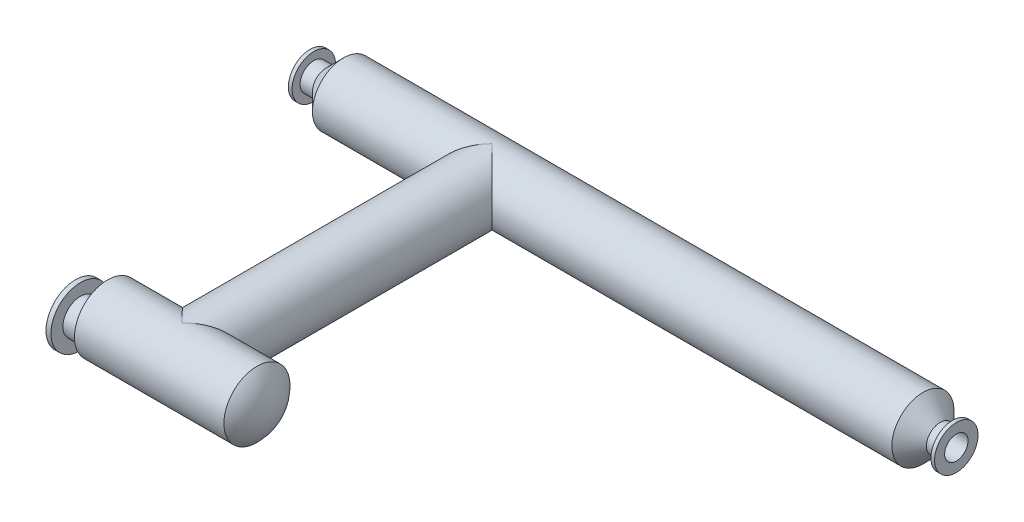
SolidWorks part; units mm, degrees
material "普通碳钢"
ref_plane "Front Plane" through (0, 0, 0) normal (0, 0, 1) x (1, 0, 0)
ref_plane "Top Plane" through (0, 0, 0) normal (0, 1, 0) x (1, 0, 0)
ref_plane "Right Plane" through (0, 0, 0) normal (1, 0, 0) x (0, 0, -1)
sketch "Sketch1" plane through (0, 0, 0) normal (0, 0, 1) x (1, 0, 0)
  line L0 (0, 56.5) -> (0, 105)
  line L1 (0, 105) -> (18, 105)
  line L2 (18, 105) -> (18, 66.5)
  line L3 (18, 66.5) -> (78, 66.5)
  line L4 (78, 66.5) -> (161.5, 150)
  line L5 (161.5, 150) -> (2962.5, 150)
  line L6 (2962.5, 150) -> (3046, 66.5)
  line L7 (3046, 66.5) -> (3106, 66.5)
  line L8 (3106, 66.5) -> (3106, 105)
  line L9 (3106, 105) -> (3124, 105)
  line L10 (3124, 105) -> (3124, 56.5)
  line L11 (3124, 56.5) -> (3041.8579, 56.5)
  line L12 (3041.8579, 56.5) -> (2958.3579, 140)
  line L13 (2958.3579, 140) -> (165.6421, 140)
  line L14 (165.6421, 140) -> (82.1421, 56.5)
  line L15 (82.1421, 56.5) -> (0, 56.5)
  line L16 (0, 0) -> (508.1939, 0) construction
  dimension "D1" = 3124
  dimension "D2" = 105
  dimension "D3" = 150
  dimension "D4" = 66.5
  dimension "D5" = 10
  dimension "D6" = 45
  dimension "D7" = 18
  dimension "D8" = 18
  dimension "D9" = 10
  dimension "D10" = 10
  dimension "D11" = 60
  dimension "D12" = 60
  dimension "D13" = 45
  dimension "D14" = 10
  dimension "D15" = 10
revolve "Revolve1" add sketch "Sketch1" angle 360 about L16
sketch "Sketch2" plane through (0, 0, 0) normal (0, 0, 1) x (1, 0, 0)
  line L0 (0, 105) -> (0, -105) construction
  circle A0 centre (880, 0) radius 150
  circle A1 centre (880, 0) radius 140
  dimension "D1" = 300
  dimension "D2" = 10
  dimension "D3" = 880
extrude "Boss-Extrude1" add sketch "Sketch2" along normal blind 1500
sketch "Sketch3" plane through (0, 0, 0) normal (-1, 0, 0) x (0, 0, 1)
  line L0 (0, 0) -> (105, 0) construction
  line L1 (0, 0) -> (0, -105) construction
  circle A0 centre (0, 0) radius 105 construction
ref_plane "Plane1" through (0, 0, 1500) normal (0, 0, 1) x (1, 0, 0)
sketch "Sketch4" plane through (0, 0, 1500) normal (0, 0, 1) x (1, 0, 0)
  line L1 (1243.1971, 150) -> (520.75, 150)
  line L2 (2962.5, 150) -> (880, 150) construction
  line L3 (880, 150) -> (161.5, 150) construction
  line L4 (497.2006, -9.7733) -> (507.2017, -9.7733)
  line L8 (1239.1001, 140) -> (528.3417, 140)
  line L10 (507.4306, 0.2267) -> (1299.0758, 0.2267) construction
  line L11 (1299.1068, -9.7733) -> (1309.109, -9.7733)
  line L12 (497.2006, -9.7733) -> (1309.109, -9.7733) construction
  arc A1 (1309.109, -9.7733) -> (1243.1971, 150) centre (1093.0729, -5.4133) ccw
  arc A2 (497.2006, -9.7733) -> (520.75, 150) centre (1110.7572, -18.5847) cw
  arc A3 (507.2017, -9.7733) -> (528.3417, 140) centre (1110.7572, -18.5847) cw
  arc A4 (1299.1068, -9.7733) -> (1239.1001, 140) centre (1093.0729, -5.4133) ccw
  arc A5 (507.4306, 0.2267) -> (528.3417, 140) centre (1110.7572, -18.5847) cw construction
  arc A6 (1299.0758, 0.2267) -> (1239.1001, 140) centre (1093.0729, -5.4133) ccw construction
  dimension "D2" = 10
revolve "Revolve2" add sketch "Sketch4" angle 360 about L4
ref_plane "Plane2" through (550, 0, 0) normal (1, 0, 0) x (0, 0, -1)
sketch "Sketch5" plane through (550, 0, 0) normal (1, 0, 0) x (0, 0, -1)
  circle A0 centre (-1559.9921, -8.8002) radius 85
  circle A1 centre (-1559.9921, -8.8002) radius 75
  circle A2 centre (-1500, -9.7733) radius 159.7733 construction
  dimension "D1" = 170
  dimension "D2" = 10
  dimension "D3" = 60
extrude "Boss-Extrude2" add sketch "Sketch5" against normal blind 100 separate body
sketch "Sketch6" plane through (450, 0, 0) normal (-1, 0, 0) x (0, 0, 1)
  circle A0 centre (1559.9921, -8.8002) radius 60.5
  circle A1 centre (1559.9921, -8.8002) radius 142.5
  dimension "D1" = 285
extrude "Boss-Extrude3" add sketch "Sketch6" along normal blind 24
